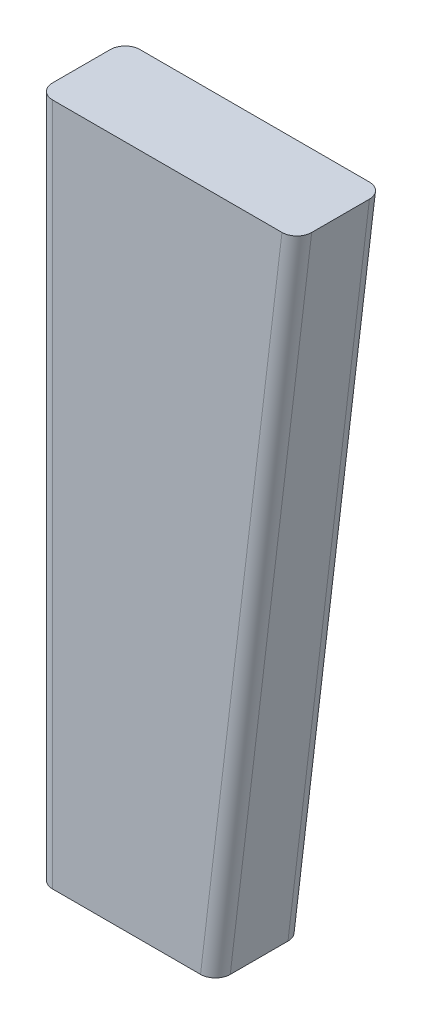
from build123d import *

# Parameters (mm, degrees)
BOSS_EXTRUDE1_DEPTH = 118
FILLET1_R           = 20


with BuildPart() as part:
    # Sketch1 → Boss-Extrude1 (new body)
    with BuildSketch(Plane.XY):
        Polygon((0, 0), (240, 0), (350, 923), (0, 923), align=None)
    extrude(amount=BOSS_EXTRUDE1_DEPTH)

    # Fillet1
    fillet1_edges = [part.edges().sort_by_distance(p)[0] for p in [
        (295, 461.5, 118),
        (0, 461.5, 118),
        (295, 461.5, 0),
        (0, 461.5, 0),
    ]]
    fillet(fillet1_edges, radius=FILLET1_R)


solid = part.part
